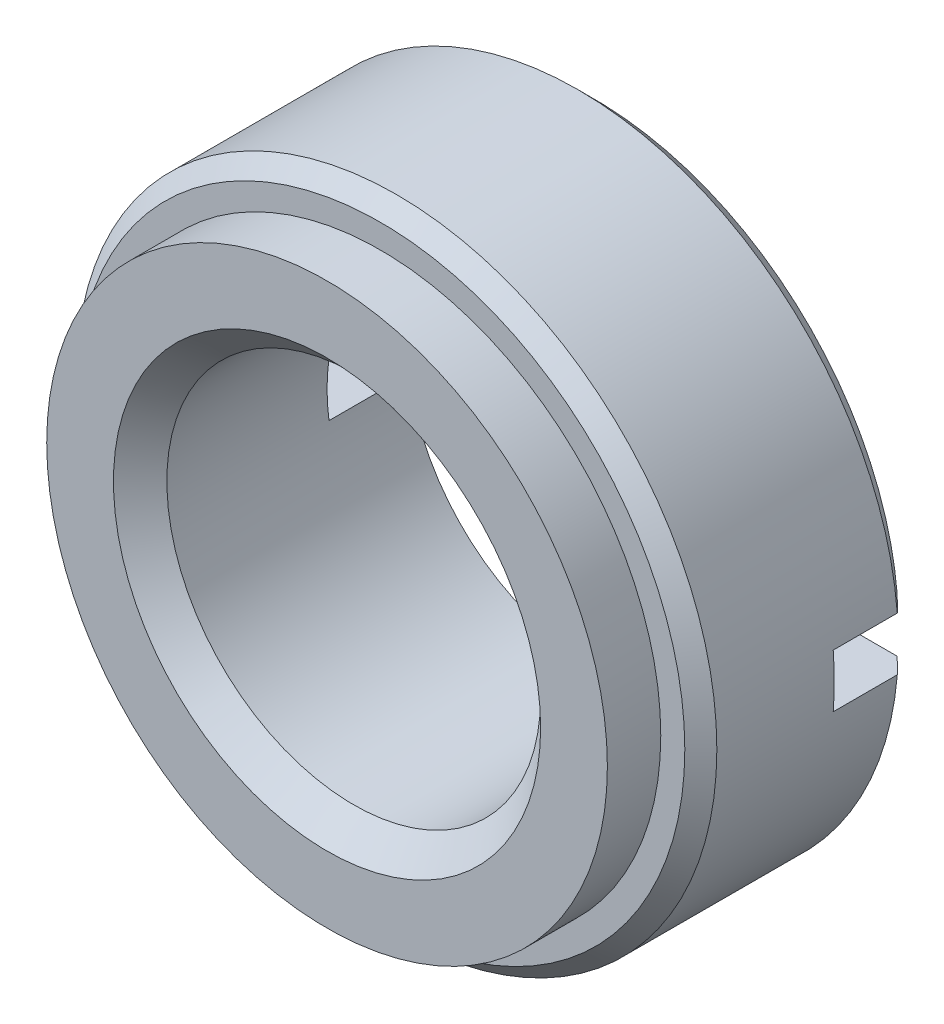
from build123d import *

# Parameters (mm, degrees)
SKETCH_1_R          = 6
SKETCH_1_R_2        = 3.5
EXTRUDE_1_DEPTH     = 5
CHAMFER_1_SIZE      = 0.5
SKETCH_2_W          = 16.841160442
SKETCH_2_H          = 1
CUT_EXTRUDE_1_DEPTH = 1.5
CUT_EXTRUDE_START   = -1
SKETCH_3_R          = 6
SKETCH_3_R_2        = 5.25
CUT_EXTRUDE_2_DEPTH = 1
CHAMFER_2_SIZE      = 0.3


with BuildPart() as part:
    # 草图1 → 凸台-拉伸1 (new body)
    with BuildSketch(Plane.XY):
        Circle(SKETCH_1_R)
        Circle(SKETCH_1_R_2, mode=Mode.SUBTRACT)
    extrude(amount=EXTRUDE_1_DEPTH)

    # 倒角1
    chamfer_1_edges = [part.edges().sort_by_distance(p)[0] for p in [
        (-3.5, 0, 5),
    ]]
    chamfer(chamfer_1_edges, length=CHAMFER_1_SIZE)

    # 草图2 → 切除-拉伸1 (cut)
    with BuildSketch(Plane(origin=(0, 0, 0), x_dir=(-1, 0, 0), z_dir=(0, 0, -1))):
        with Locations((-0.328074554, 0)):
            Rectangle(SKETCH_2_W, SKETCH_2_H)
    extrude(amount=-CUT_EXTRUDE_1_DEPTH, mode=Mode.SUBTRACT)

    # 草图3 → 切除-拉伸2 (cut)
    with BuildSketch(Plane.XY.offset(5).offset(CUT_EXTRUDE_START)):
        with Locations(Location((0, 0, 0), (0, 0, 175.219808153))):
            Circle(SKETCH_3_R)
        Circle(SKETCH_3_R_2, mode=Mode.SUBTRACT)
    extrude(amount=CUT_EXTRUDE_2_DEPTH, mode=Mode.SUBTRACT)

    # 倒角2
    chamfer_2_edges = [part.edges().sort_by_distance(p)[0] for p in [
        (0, -6, 0),
        (0, 6, 0),
        (-6, 0, 4),
    ]]
    chamfer(chamfer_2_edges, length=CHAMFER_2_SIZE)


solid = part.part
